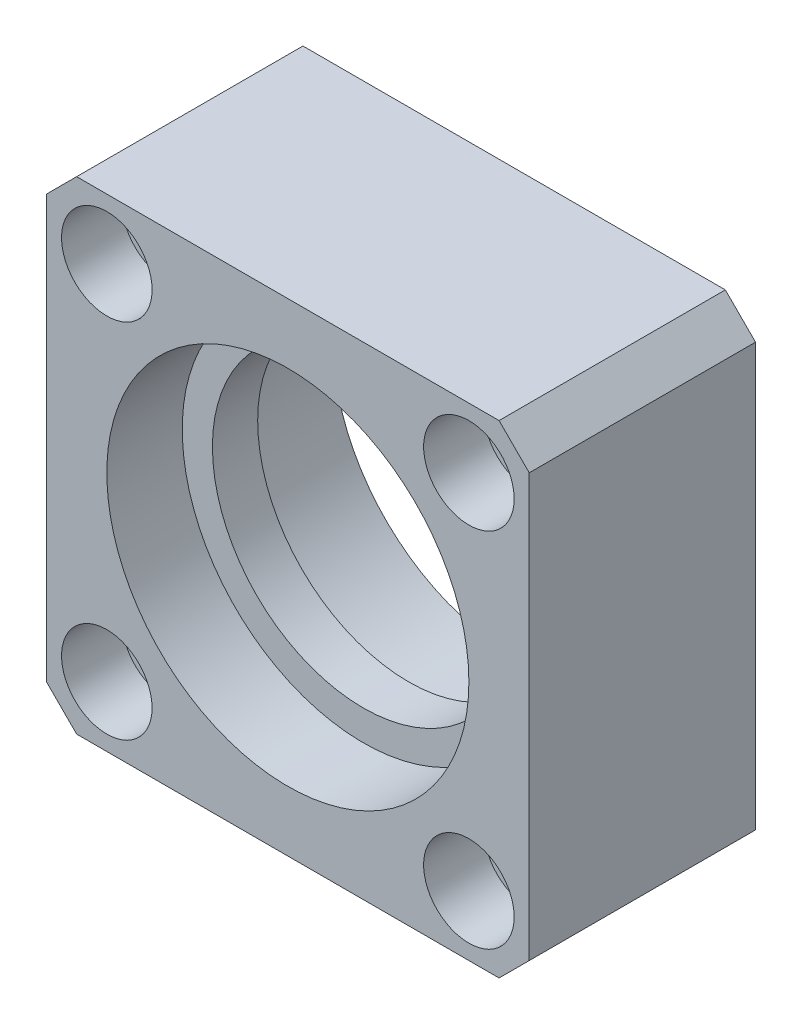
from build123d import *

# Parameters (mm, degrees)
SKETCH1_W                                            = 32
SKETCH1_H                                            = 32
BOSS_EXTRUDE1_DEPTH                                  = 7.5
SKETCH2_R                                            = 10
CUT_EXTRUDE1_DEPTH                                   = 28.147743921
SKETCH3_R                                            = 12
CUT_EXTRUDE2_DEPTH                                   = 5
CUT_EXTRUDE3_START                                   = -7
SKETCH4_R                                            = 12
CUT_EXTRUDE3_DEPTH                                   = 7
CHAMFER1_SIZE                                        = 2
HOLE_SIZE_PER_SOCKET_HEAD_CAP_SCREW_TYPE_D           = 3.5
HOLE_SIZE_PER_SOCKET_HEAD_CAP_SCREW_TYPE_CBORE_D     = 6
HOLE_SIZE_PER_SOCKET_HEAD_CAP_SCREW_TYPE_CBORE_DEPTH = 4


with BuildPart() as part:
    # Sketch1 → Boss-Extrude1 (new, symmetric)
    with BuildSketch(Plane.XY):
        Rectangle(SKETCH1_W, SKETCH1_H)
    extrude(amount=BOSS_EXTRUDE1_DEPTH, both=True)

    # Sketch2 → Cut-Extrude1 (cut, through all)
    with BuildSketch(Plane.XY.offset(7.5)):
        Circle(SKETCH2_R)
    extrude(amount=-CUT_EXTRUDE1_DEPTH, mode=Mode.SUBTRACT)

    # Sketch3 → Cut-Extrude2 (cut)
    with BuildSketch(Plane.XY.offset(7.5)):
        Circle(SKETCH3_R)
    extrude(amount=-CUT_EXTRUDE2_DEPTH, mode=Mode.SUBTRACT)

    # Sketch4 → Cut-Extrude3 (cut)
    with BuildSketch(Plane(origin=(0, 0, -7.5), x_dir=(-1, 0, 0), z_dir=(0, 0, -1)).offset(CUT_EXTRUDE3_START)):
        with Locations(Location((0, 0, 0), (0, 0, 180))):
            Circle(SKETCH4_R)
    extrude(amount=CUT_EXTRUDE3_DEPTH, mode=Mode.SUBTRACT)

    # Chamfer1
    chamfer1_edges = [part.edges().sort_by_distance(p)[0] for p in [
        (16, -16, 0),
        (-16, -16, 0),
        (-16, 16, 0),
        (16, 16, 0),
    ]]
    chamfer(chamfer1_edges, length=CHAMFER1_SIZE)

    # Hole size per socket head cap screw type1 (through all)
    with Locations(Plane.XY.offset(7.5)):
        with Locations((-12, 12), (12, 12), (12, -12), (-12, -12)):
            CounterBoreHole(HOLE_SIZE_PER_SOCKET_HEAD_CAP_SCREW_TYPE_D / 2, HOLE_SIZE_PER_SOCKET_HEAD_CAP_SCREW_TYPE_CBORE_D / 2, HOLE_SIZE_PER_SOCKET_HEAD_CAP_SCREW_TYPE_CBORE_DEPTH)


solid = part.part
